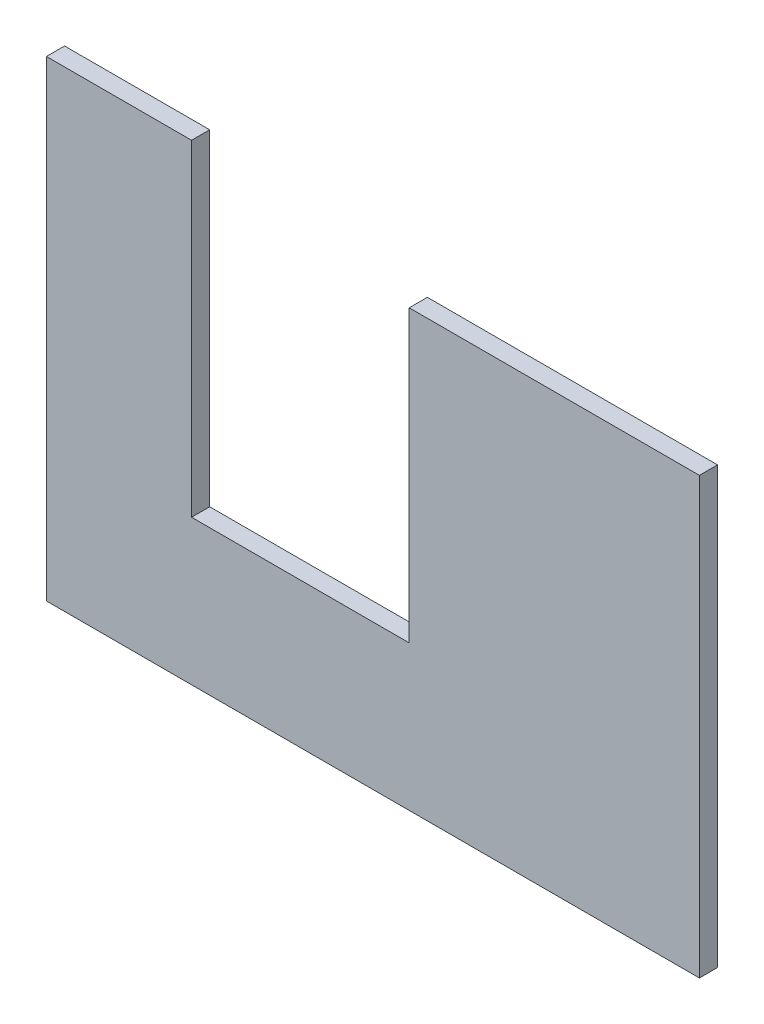
SolidWorks part; units mm, degrees
ref_plane "前视基准面" through (0, 0, 0) normal (0, 0, 1) x (1, 0, 0)
ref_plane "上视基准面" through (0, 0, 0) normal (0, 1, 0) x (1, 0, 0)
ref_plane "右视基准面" through (0, 0, 0) normal (1, 0, 0) x (0, 0, -1)
sketch "草图1" plane through (0, 0, 0) normal (0, 0, 1) x (1, 0, 0)
  line L0 (0, 0) -> (0, 130)
  line L1 (0, 130) -> (40, 130)
  line L2 (0, 0) -> (180, 0)
  line L3 (180, 0) -> (180, 120)
  line L4 (180, 120) -> (100, 120)
  line L7 (100, 40) -> (40, 40)
  line L8 (40, 130) -> (40, 40)
  line L9 (100, 40) -> (100, 120)
extrude "凸台-拉伸1" add sketch "草图1" along normal blind 5
